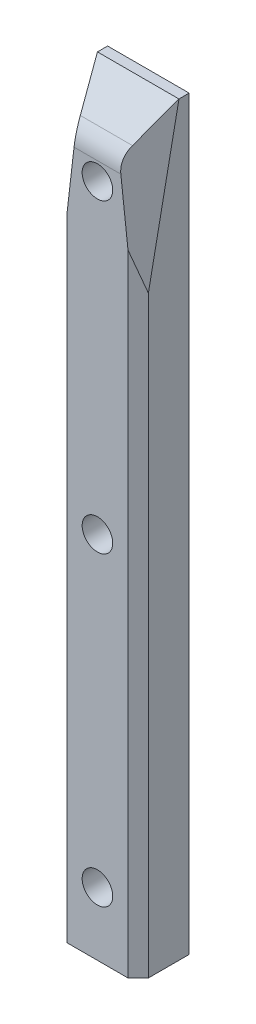
SolidWorks part; units mm, degrees
material "PC"
ref_plane "Front Plane" through (0, 0, 0) normal (0, 0, 1) x (1, 0, 0)
ref_plane "Top Plane" through (0, 0, 0) normal (0, 1, 0) x (1, 0, 0)
ref_plane "Right Plane" through (0, 0, 0) normal (1, 0, 0) x (0, 0, -1)
sketch "Sketch1" plane through (0, 0, 0) normal (0, 0, 1) x (1, 0, 0)
  line L1 (-20, 183) -> (20, 183)
  line L2 (-20, 183) -> (-20, -183)
  line L3 (-20, -183) -> (20, -183)
  line L4 (20, 183) -> (20, -183)
  line L5 (-20, 183) -> (20, -183) construction
  line L6 (-20, -183) -> (20, 183) construction
  point P0 (0, 0)
  dimension "D1" = 40
  dimension "D2" = 366
extrude "Boss-Extrude1" add sketch "Sketch1" along normal blind 25
chamfer "Chamfer1" [suppressed] distance 20 angle 30
hole_wizard "M6 Tapped Hole1" positions "Sketch2" profile "Sketch3" tap size "M6" standard "GB"
sketch "Sketch2" plane through (0, 0, 0) normal (0, 0, -1) x (-1, 0, 0)
  line L0 (0, 150) -> (0, 175) construction
  line L1 (-20, 175) -> (20, 175) construction
  line L6 (20, -175) -> (-20, -175) construction
  point P0 (0, 150)
  point P5 (0, -150)
  point P19 (0, 0)
  dimension "D1" = 25
  dimension "D2" = 150
  dimension "D3" = 150
sketch "Sketch3" plane through (0, 150, 0) normal (1, 0, 0) x (0, 1, 0)
  line L0 (0, 0) -> (0, 27)
  line L1 (0, 27) -> (2.5, 27)
  line L2 (2.5, 27) -> (2.5, 0)
  line L5 (2.5, 0) -> (0, 0)
  line L11 (0, -6.35) -> (0, 107.95) construction
  dimension "通孔螺纹孔钻头直径" = 5
  dimension "通孔螺纹孔钻头深度" = 27
cosmetic thread "Cosmetic Thread1" [suppressed] parameters "D2"=6
cosmetic thread "Cosmetic Thread2" [suppressed] parameters "D2"=6
cosmetic thread "Cosmetic Thread3" [suppressed] parameters "D2"=6
chamfer "Chamfer2" [suppressed] distance 20 angle 22.5
sketch "Sketch4" plane through (0, 0, 25) normal (0, 0, 1) x (1, 0, 0)
  line L0 (0, -183) -> (0, -152) construction
  line L1 (-20, -183) -> (20, -183) construction
  circle A0 centre (0, -152) radius 7.5
  circle A1 centre (0, -2) radius 7.5
  circle A2 centre (0, 148) radius 7.5
  dimension "D1" = 15
  dimension "D2" = 31
  dimension "D3" = 150
  dimension "D4" = 150
extrude "Cut-Extrude1" cut sketch "Sketch4" against normal blind 2
hole_wizard "Hole Size (based on) hex socket cap screw type 1" positions "Sketch5" profile "Sketch6" counterbore size "M8" standard "GB" end condition through all
sketch "Sketch5" plane through (0, 0, 23) normal (0, 0, 1) x (1, 0, 0)
  point P0 (0, -152)
  point P3 (0, -2)
  point P6 (0, 148)
sketch "Sketch6" plane through (0, -152, 23) normal (1, 0, 0) x (0, -1, 0)
  line L0 (0, 0) -> (0, 23)
  line L1 (0, 23) -> (4.5, 23)
  line L3 (4.5, 23) -> (4.5, 10)
  line L4 (4.5, 10) -> (7.5, 10)
  line L5 (7.5, 10) -> (7.5, 0)
  line L7 (7.5, 0) -> (0, 0)
  line L11 (0, -6.35) -> (0, 107.95) construction
  dimension "通孔孔直径" = 9
  dimension "通孔孔深度" = 23
  dimension "柱形沉头孔直径" = 15
  dimension "柱形沉头孔深度" = 10
sketch "Sketch7" plane through (0, 0, 25) normal (0, 0, 1) x (1, 0, 0)
  line L0 (-20, -179) -> (15, -183)
  line L1 (-20, 183) -> (-20, -183) construction
  line L2 (-20, -183) -> (20, -183) construction
  line L3 (15, -183) -> (-20, -183)
  line L4 (-20, -183) -> (-20, -179)
  dimension "D1" = 35
  dimension "D2" = 4
extrude "Cut-Extrude2" [suppressed] cut sketch "Sketch7" against normal through all
fillet "Fillet1" [suppressed] radius 5
sketch "Sketch8" [suppressed] plane through (0, 0, 25) normal (0, 0, 1) x (1, 0, 0)
  line L0 (-15, -183) -> (20, -179)
  line L1 (-15, -183) -> (15, -183) construction
  line L2 (20, 160.9289) -> (20, -183) construction
  line L3 (20, -179) -> (20, -183)
  line L4 (20, -183) -> (-15, -183)
  dimension "D1" = 35
  dimension "D2" = 4
extrude "Cut-Extrude3" [suppressed] cut sketch "Sketch8" against normal through all
chamfer "Chamfer3" [suppressed] distance 5 angle 45
fillet "Fillet2" [suppressed] radius 15
sketch "Sketch9" plane through (-20, 0, 0) normal (-1, 0, 0) x (0, 0, 1)
  line L0 (5, 183) -> (25, 83)
  line L1 (25, 183) -> (0, 183) construction
  line L2 (25, 183) -> (25, -183) construction
  dimension "D1" = 5
  dimension "D2" = 100
sketch "Sketch10" plane through (0, 183, 0) normal (0, 1, 0) x (1, 0, 0)
  line L0 (-20, -5) -> (-8.453, -25)
  line L1 (-20, -25) -> (-20, 0) construction
  line L2 (-20, -5) -> (-20, -25) construction
  line L3 (20, -25) -> (-20, -25) construction
  dimension "D1" = 30
sketch "Sketch11" plane through (0, 0, 25) normal (0, 0, 1) x (1, 0, 0)
  line L0 (-20, 83) -> (-8.453, 183)
  line L1 (-20, 183) -> (-20, 83) construction
  line L2 (-20, 183) -> (-20, -183) construction
  dimension "D1" = 100
ref_plane "Plane1" through (-32.6865, 3.7743, 18.8715) normal (-0.8617, 0.0995, 0.4975) x (0.4686, -0.2201, 0.8556)
sketch "Sketch13" plane through (-32.6865, 3.7743, 18.8715) normal (-0.8617, 0.0995, 0.4975) x (0.4686, -0.2201, 0.8556)
  line L0 (-6.25, 80.2256) -> (-22.8497, 179.512) construction
  line L1 (-6.25, 80.2256) -> (-22.8497, 179.512)
  line L2 (-45.3717, 174.4036) -> (-22.8497, 179.512) construction
  line L3 (-45.3717, 174.4036) -> (-22.8497, 179.512)
  line L4 (-45.3717, 174.4036) -> (-6.25, 80.2256) construction
  line L5 (-45.3717, 174.4036) -> (-6.25, 80.2256)
extrude "Cut-Extrude4" cut sketch "Sketch13" along normal blind 15
ref_plane "Plane2" through (0, 0, 0) normal (-1, 0, 0) x (0, 0, 1)
mirror "Mirror1" about plane through (0, 0, 0) normal (-1, 0, 0) of "Cut-Extrude4"
chamfer "Chamfer4" distance 5 angle 45 2 edges at (20, -50, 25) (-20, -50, 25)
chamfer "Chamfer5" [suppressed] distance 5 angle 45
sketch "Sketch14" plane through (-20, 0, 0) normal (-1, 0, 0) x (0, 0, 1)
  line L0 (5, 183) -> (25, 163)
  line L1 (25, 126.3013) -> (25, 183) construction
  line L2 (25, 163) -> (25, 183)
  line L3 (25, 183) -> (5, 183)
  dimension "D1" = 20
extrude "Cut-Extrude5" cut sketch "Sketch14" against normal through all
fillet "Fillet3" radius 15 1 edges at (0, 163, 25)
